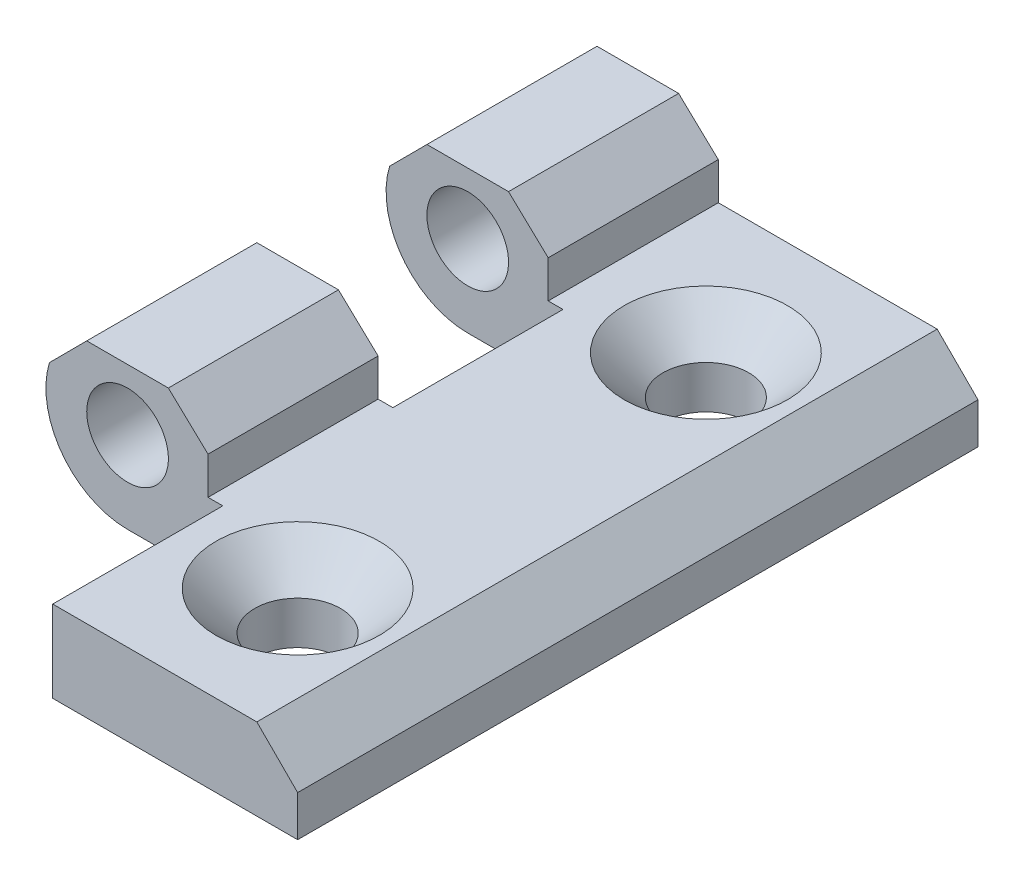
SolidWorks part; units mm, degrees
material "AISI 304"
ref_plane "前视基准面" through (0, 0, 0) normal (0, 0, 1) x (1, 0, 0)
ref_plane "上视基准面" through (0, 0, 0) normal (0, 1, 0) x (1, 0, 0)
ref_plane "右视基准面" through (0, 0, 0) normal (1, 0, 0) x (0, 0, -1)
sketch "草图1" plane through (0, 0, 0) normal (0, 0, 1) x (1, 0, 0)
  line L0 (-7, 1) -> (0, 1)
  line L1 (0, 0) -> (18, 0)
  line L2 (0, 0) -> (0, 1)
  line L3 (-1.0839, 6) -> (18, 6)
  line L4 (18, 0) -> (18, 6)
  line L5 (-25.1126, 11.5) -> (12, 11.5) construction
  line L6 (-10, 11.5) -> (-4, 11.5)
  line L7 (-12.7396, 8.7483) -> (-10, 11.5)
  line L8 (-1.0839, 6) -> (-1.0839, 8.7483)
  line L9 (-1.0839, 8.7483) -> (-4, 11.5)
  line L10 (-4, 11.5) -> (-4.0054, 11.4989)
  line L11 (-7, 7) -> (-7, 2.5125) construction
  line L12 (-1.0839, 8.7483) -> (-18.3005, 8.7483) construction
  circle A0 centre (-7, 7) radius 3
  arc A1 (-12.7396, 8.7483) -> (-7, 1) centre (-7, 7) ccw
  circle A2 centre (-7, 7) radius 6 construction
  dimension "D3" = 6
  dimension "D5" = 25
  dimension "D8" = 1
  dimension "D1" = 18
  dimension "D2" = 6
  dimension "D6" = 11.5
  dimension "D7" = 6
  dimension "D4" = 3
extrude "拉伸1" add sketch "草图1" along normal mid plane 50
chamfer "倒角1" distance 3 angle 45 1 edges at (18, 6, 0)
sketch "草图2" plane through (0, 6, 0) normal (0, 1, 0) x (1, 0, 0)
  line L0 (18, 0) -> (-23.467, 0) construction
  line L1 (18, 25) -> (18, -25) construction
  circle A0 centre (8, 15) radius 1.0721
  circle A1 centre (8, -15) radius 1.0721
  dimension "D1" = 30
  dimension "D2" = 10
extrude "切除-拉伸1" cut sketch "草图2" against normal blind 50
hole_wizard "打孔尺寸开槽半沉头螺钉的类型1" positions "3D草图1" profile "草图3" countersink size "M6" standard "GB" end condition through all
sketch3d "3D草图1"
  line L0 (8, 0, -15) -> (8, 6, -15) construction
  line L1 (8, 0, 15) -> (8, 6, 15) construction
  point P0 (8, 6, -15)
  point P4 (8, 6, 15)
sketch "草图3" plane through (8, 6, -15) normal (1, 0, 0) x (0, 0, 1)
  line L0 (0, 0) -> (0, 6)
  line L1 (0, 6) -> (3.15, 6)
  line L2 (3.15, 6) -> (3.15, 2.85)
  line L3 (3.15, 2.85) -> (6, 0)
  line L5 (6, 0) -> (0, 0)
  line L6 (-3.15, 2.85) -> (-6, 0) construction
  line L11 (0, -6.35) -> (0, 107.95) construction
  dimension "籵謂謂眻噤" = 6.3
  dimension "籵謂謂旮僅" = 6
  dimension "輪傷袪倛麥芛謂眻噤" = 12
  dimension "輪傷袪倛麥芛謂褒僅" = 90
sketch "草图4" plane through (0, 11.5, 0) normal (0, 1, 0) x (1, 0, 0)
  line L1 (18, 25) -> (18, -25) construction
  line L2 (-23.8811, 0) -> (0, 0)
  line L3 (-23.8811, 0) -> (-23.8811, 12.5)
  line L4 (-23.8811, 12.5) -> (0, 12.5)
  line L5 (0, 0) -> (0, 12.5)
  line L6 (-1.0839, 25) -> (15, 25) construction
  line L8 (-26.9107, -12.5) -> (0, -12.5)
  line L9 (-26.9107, -12.5) -> (-26.9107, -25)
  line L10 (-26.9107, -25) -> (0, -25)
  line L11 (0, -12.5) -> (0, -25)
  point P6 (6.958, 25)
  dimension "D1" = 18
  dimension "D2" = 12.5
  dimension "D3" = 12.5
  dimension "D4" = 12.5
  dimension "D5" = 12.5
extrude "切除-拉伸2" cut sketch "草图4" against normal blind 50
